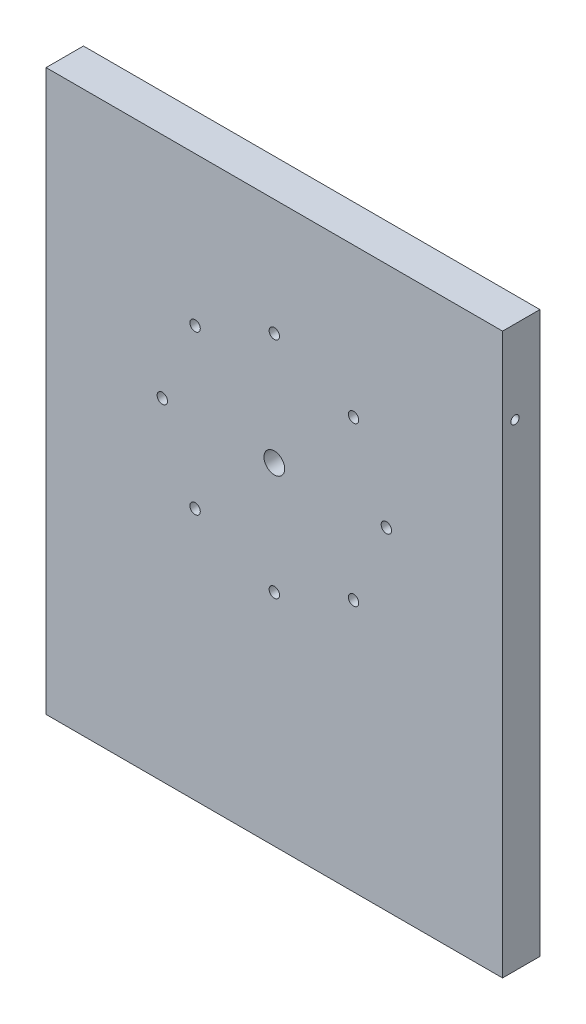
from build123d import *

# Parameters (mm, degrees)
SKETCH_1_W          = 220
SKETCH_1_H          = 280
EXTRUDE_1_DEPTH     = 18
SKETCH_2_W          = 220
SKETCH_2_H          = 60
CUT_EXTRUDE_1_DEPTH = 179.952507666
SKETCH_4_R          = 5
CUT_EXTRUDE_3_DEPTH = 179.952507666
SKETCH_5_R          = 2.5
CUT_EXTRUDE_4_DEPTH = 179.952507666
SKETCH_13_W         = 18
SKETCH_13_H         = 50
EXTRUDE_2_DEPTH     = 220
SKETCH_15_R         = 2
CUT_EXTRUDE_5_DEPTH = 262.388599598


with BuildPart() as part:
    # 草图1 → 凸台-拉伸1 (new body)
    with BuildSketch(Plane.XY):
        Rectangle(SKETCH_1_W, SKETCH_1_H)
    extrude(amount=EXTRUDE_1_DEPTH)

    # 草图2 → 切除-拉伸1 (cut, through all)
    with BuildSketch(Plane.XY):
        with Locations((0, -110)):
            Rectangle(SKETCH_2_W, SKETCH_2_H)
    extrude(amount=CUT_EXTRUDE_1_DEPTH, mode=Mode.SUBTRACT)

    # 草图4 → 切除-拉伸3 (cut, through all)
    with BuildSketch(Plane.XY):
        with Locations((0, 30)):
            Circle(SKETCH_4_R)
    extrude(amount=CUT_EXTRUDE_3_DEPTH, mode=Mode.SUBTRACT)

    # 草图5 → 切除-拉伸4 (cut, through all)
    with BuildSketch(Plane(origin=(0, 0, 0), x_dir=(-1, 0, 0), z_dir=(0, 0, -1))):
        with Locations((-38.183766184, 68.183766184)):
            Circle(SKETCH_5_R)
        with Locations((0, 84)):
            Circle(SKETCH_5_R)
        with Locations((-54, 30)):
            Circle(SKETCH_5_R)
        with Locations((-38.183766184, -8.183766184)):
            Circle(SKETCH_5_R)
        with Locations((0, -24)):
            Circle(SKETCH_5_R)
        with Locations((38.183766184, -8.183766184)):
            Circle(SKETCH_5_R)
        with Locations((54, 30)):
            Circle(SKETCH_5_R)
        with Locations((38.183766184, 68.183766184)):
            Circle(SKETCH_5_R)
    extrude(amount=-CUT_EXTRUDE_4_DEPTH, mode=Mode.SUBTRACT)

    # 草图13 → 凸台-拉伸2 (add, through all)
    with BuildSketch(Plane.ZY.offset(110)):
        with Locations((9, -105)):
            Rectangle(SKETCH_13_W, SKETCH_13_H)
    extrude(amount=-EXTRUDE_2_DEPTH)

    # 草图15 → 切除-拉伸5 (cut, through all)
    with BuildSketch(Plane(origin=(110, 0, 0), x_dir=(0, 0, -1), z_dir=(1, 0, 0))):
        with Locations((-12, 100)):
            Circle(SKETCH_15_R)
    extrude(amount=-CUT_EXTRUDE_5_DEPTH, mode=Mode.SUBTRACT)


solid = part.part
